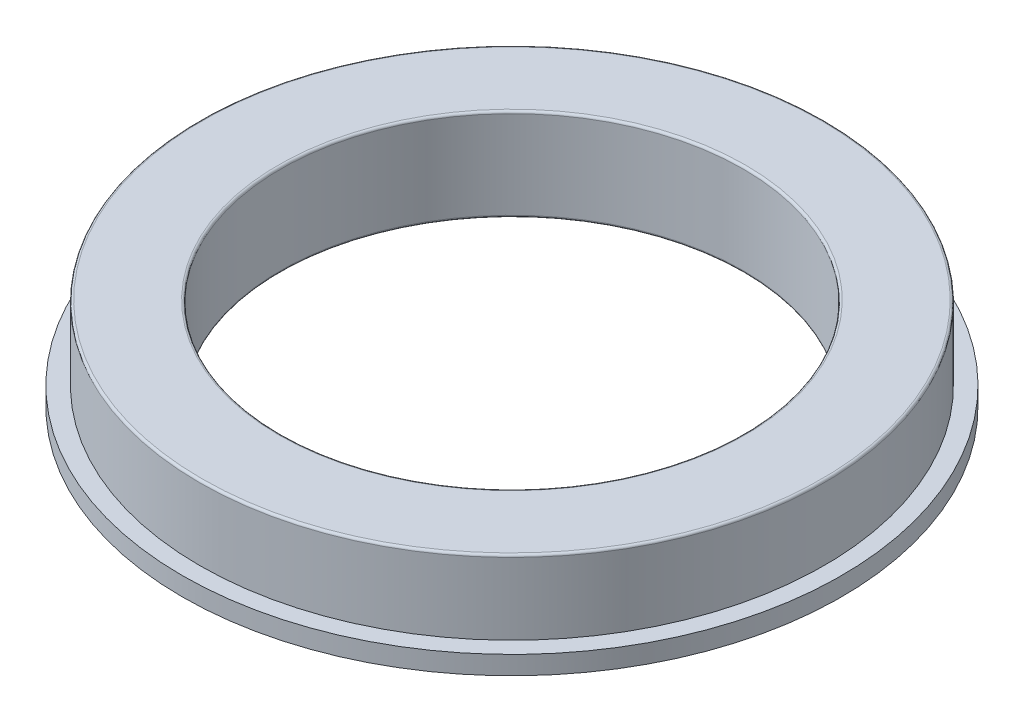
SolidWorks part; units mm, degrees
material "镀铬不锈钢"
ref_plane "前视基准面" through (0, 0, 0) normal (0, 0, 1) x (1, 0, 0)
ref_plane "上视基准面" through (0, 0, 0) normal (0, 1, 0) x (1, 0, 0)
ref_plane "右视基准面" through (0, 0, 0) normal (1, 0, 0) x (0, 0, -1)
sketch "草图1" plane through (0, 0, 0) normal (0, 1, 0) x (1, 0, 0)
  circle A0 centre (0, 0) radius 14.25
  circle A1 centre (0, 0) radius 10
  dimension "D1" = 28.5
  dimension "D2" = 20
extrude "凸台-拉伸1" add sketch "草图1" along normal blind 0.8
sketch "草图2" plane through (0, 0.8, 0) normal (0, 1, 0) x (1, 0, 0)
  circle A0 centre (0, 0) radius 13.5
  circle A1 centre (0, 0) radius 10 construction
  circle A2 centre (0, 0) radius 10
  dimension "D1" = 27
extrude "凸台-拉伸2" add sketch "草图2" along normal blind 3.2
fillet "R0.1 圆角1" radius 0.1 3 edges at (0, 0, 10) (0, 4, 10) (0, 4, 13.5)
